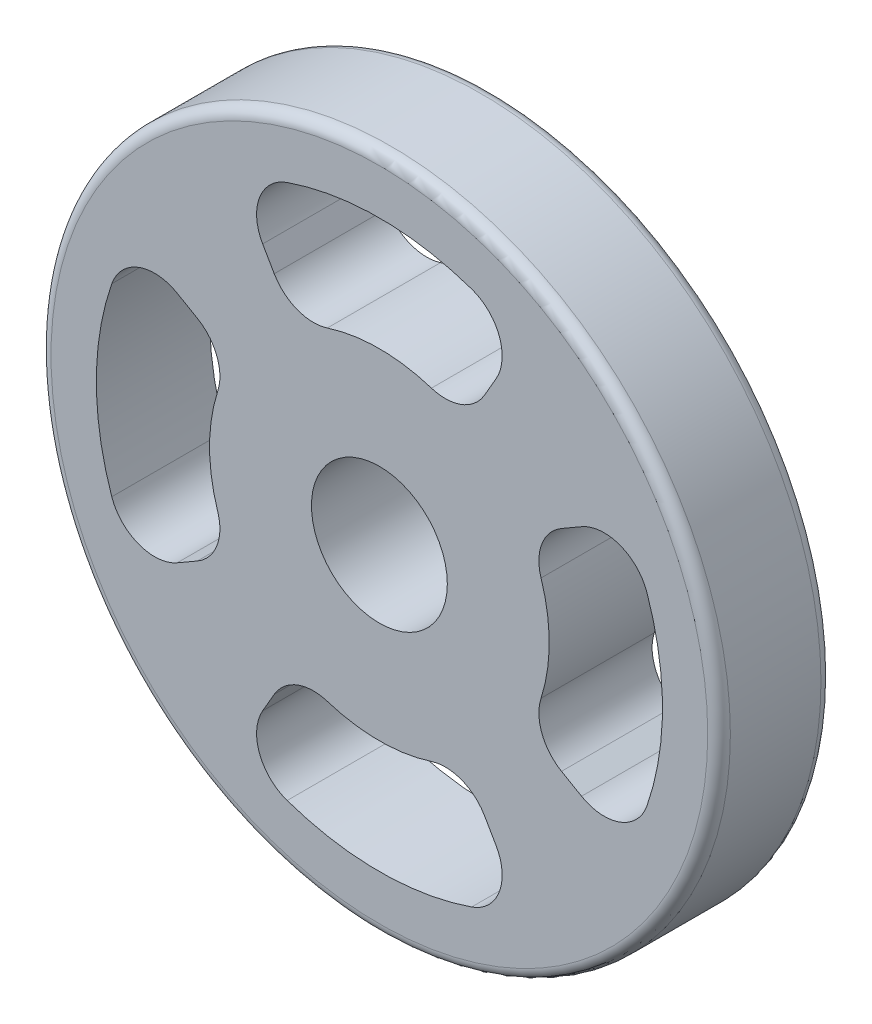
SolidWorks part; units mm, degrees
ref_plane "Front Plane" through (0, 0, 0) normal (0, 0, 1) x (1, 0, 0)
ref_plane "Top Plane" through (0, 0, 0) normal (0, 1, 0) x (1, 0, 0)
ref_plane "Right Plane" through (0, 0, 0) normal (1, 0, 0) x (0, 0, -1)
other "Configuration Table"
sketch "Sketch1" plane through (0, 0, 0) normal (0, 0, 1) x (1, 0, 0)
  circle A0 centre (0, 0) radius 15
  circle A1 centre (0, 0) radius 3
  dimension "D1" = 30
  dimension "D2" = 6
extrude "Boss-Extrude1" add sketch "Sketch1" along normal blind 5 contours A1 | A0
sketch "Sketch2" plane through (0, 0, 5) normal (0, 0, 1) x (1, 0, 0)
  line L0 (-5.1539, 8.9268) -> (-4.6435, 8.0429)
  line L1 (0, 0) -> (0, 9.1767) construction
  line L2 (5.1539, 8.9268) -> (4.6435, 8.0429)
  line L3 (8.9268, 5.1539) -> (8.0429, 4.6435)
  line L4 (8.9268, -5.1539) -> (8.0429, -4.6435)
  line L5 (5.1539, -8.9268) -> (4.6435, -8.0429)
  line L6 (-5.1539, -8.9268) -> (-4.6435, -8.0429)
  line L7 (-8.9268, -5.1539) -> (-8.0429, -4.6435)
  line L8 (-8.9268, 5.1539) -> (-8.0429, 4.6435)
  arc A0 (4.0736, 11.8176) -> (-4.0736, 11.8176) centre (0, 0) ccw
  arc A1 (-4.6435, 8.0429) -> (-2.2985, 7.1391) centre (-2.9115, 9.0429) ccw
  arc A3 (2.2985, 7.1391) -> (-2.2985, 7.1391) centre (0, 0) ccw
  arc A4 (4.6435, 8.0429) -> (2.2985, 7.1391) centre (2.9115, 9.0429) cw
  arc A5 (5.1539, 8.9268) -> (4.0736, 11.8176) centre (3.4218, 9.9268) ccw
  arc A6 (-5.1539, 8.9268) -> (-4.0736, 11.8176) centre (-3.4218, 9.9268) cw
  arc A7 (8.9268, -5.1539) -> (11.8176, -4.0736) centre (9.9268, -3.4218) ccw
  arc A8 (11.8176, -4.0736) -> (11.8176, 4.0736) centre (0, 0) ccw
  arc A9 (8.9268, 5.1539) -> (11.8176, 4.0736) centre (9.9268, 3.4218) cw
  arc A10 (8.0429, 4.6435) -> (7.1391, 2.2985) centre (9.0429, 2.9115) ccw
  arc A11 (7.1391, -2.2985) -> (7.1391, 2.2985) centre (0, 0) ccw
  arc A12 (8.0429, -4.6435) -> (7.1391, -2.2985) centre (9.0429, -2.9115) cw
  arc A13 (-5.1539, -8.9268) -> (-4.0736, -11.8176) centre (-3.4218, -9.9268) ccw
  arc A14 (-4.0736, -11.8176) -> (4.0736, -11.8176) centre (0, 0) ccw
  arc A15 (5.1539, -8.9268) -> (4.0736, -11.8176) centre (3.4218, -9.9268) cw
  arc A16 (4.6435, -8.0429) -> (2.2985, -7.1391) centre (2.9115, -9.0429) ccw
  arc A17 (-2.2985, -7.1391) -> (2.2985, -7.1391) centre (0, 0) ccw
  arc A18 (-4.6435, -8.0429) -> (-2.2985, -7.1391) centre (-2.9115, -9.0429) cw
  arc A19 (-8.9268, 5.1539) -> (-11.8176, 4.0736) centre (-9.9268, 3.4218) ccw
  arc A20 (-11.8176, 4.0736) -> (-11.8176, -4.0736) centre (0, 0) ccw
  arc A21 (-8.9268, -5.1539) -> (-11.8176, -4.0736) centre (-9.9268, -3.4218) cw
  arc A22 (-8.0429, -4.6435) -> (-7.1391, -2.2985) centre (-9.0429, -2.9115) ccw
  arc A23 (-7.1391, 2.2985) -> (-7.1391, -2.2985) centre (0, 0) ccw
  arc A24 (-8.0429, 4.6435) -> (-7.1391, 2.2985) centre (-9.0429, 2.9115) cw
  point P17 (6.25, 10.8253)
  point P20 (-6.25, 10.8253)
  dimension "D1" = 25
  dimension "D3" = 15
  dimension "D5" = 2
  dimension "D2" = 30
  dimension "D4" = 30
  dimension "D6" = 4
extrude "Cut-Extrude1" cut sketch "Sketch2" against normal blind 5
fillet "Fillet1" radius 0.5 2 edges at (15, 0, 0) (15, 0, 5)
